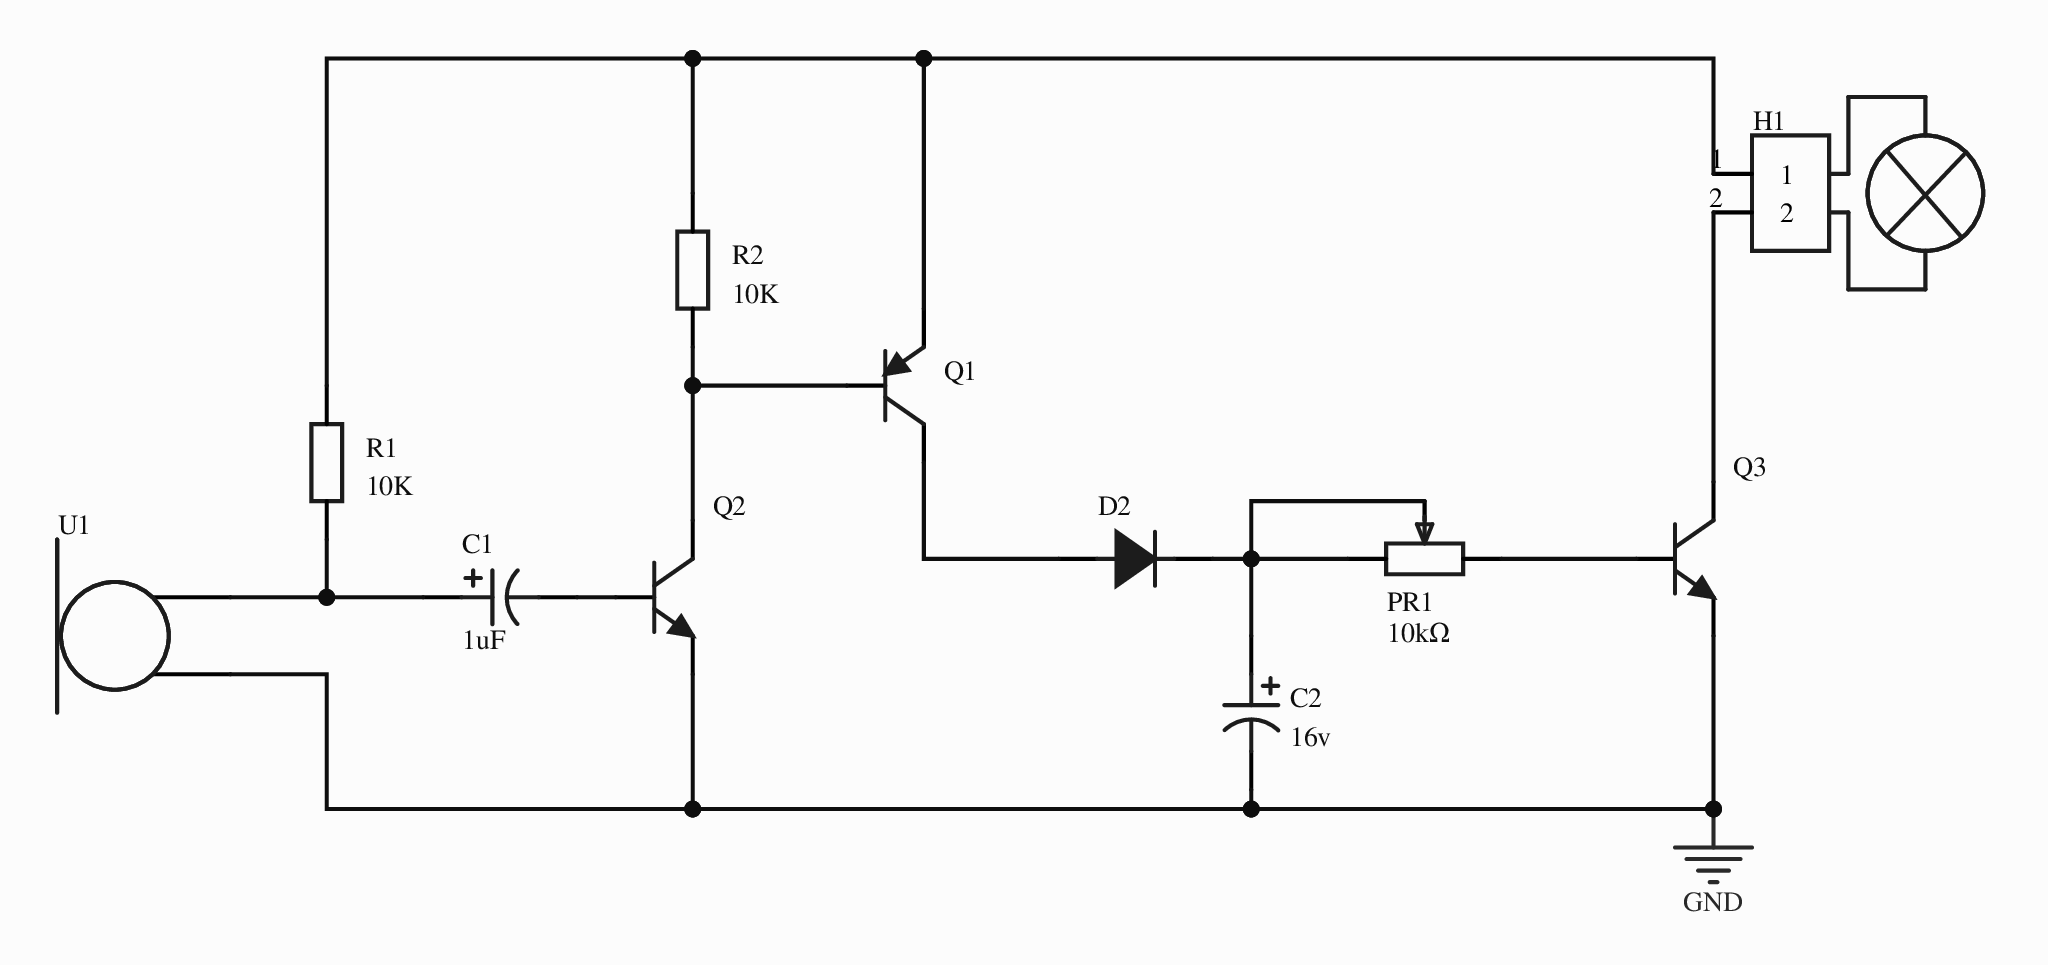
[diagram p0: MISC49923-3.schdoc]
# Altium project MISC49923-2.PrjPcb
1 sheet, 11 parts. Net scope: global (net labels, ports and power ports of the same name join across sheets).
Board file: MISC49923.pcbdoc

## Sheet MISC49923-3.schdoc
size 297 x 209 mm; Version: V1.0; @Project Name: MISC49923; @Update Date: 2026-10-05; @Create Date: 2026-10-05; @Board Name: MISC49923; @Create Time: 20:24:00; @Page Count: 1; @Page No: 1; @Schematic Name: MISC49923; @Update Time: 20:24:00; Size: A4

### Parts
C1  1uF  [CAP-TH_BD5.0-P2.00-D0.8-FD-10UF50VC110GL]
C2  16v  [CAP-TH_BD5.0-P2.00-D0.8-FD-10UF50VC110GL]
D2  (no value)  [SMA_1N4007]
H1  (no value)  [HDR-TH_2P-P2.54-V-M-1]
PR1  10kΩ  [R_3296]
Q1  (no value)  [S8550P_SOT]
Q2  (no value)  [S8050_SOT-23]
Q3  (no value)  [S8050_SOT-23]
R1  10K  [R0603]
R2  10K  [R0603]
U1  Current source  [咪头]  (value not drawn)

### Nets
GND: C2.2 Q2.2 Q3.2 U1.1
NetC1_1: C1.1 R1.1 U1.2
NetC1_2: C1.2 Q2.1
NetC2_1: C2.1 D2.1(K) PR1.2 PR1.3
NetD2_2: D2.2(A) Q1.3(C)
NetH1_1: H1.1 Q1.2(E) R1.2 R2.2
NetH1_2: H1.2 Q3.3
NetPR1_1: PR1.1 Q3.1
NetQ1_1: Q1.1(B) Q2.3 R2.1

### Library data of the parts
C1 C2 = 10UF50VC110GL: Capacitance:10uF;Tolerance:±20%;Rated voltage:50V;Ripple current:120mA@100KHz;Equivalent series resistance(ESR):1.6Ω;; Manufacturer: Econd(米朗电子); AddInBom: yes; ModelId: b35ab6b0460c4c43a629d91cfc2b58780819f05c4eef4c71ace90d822a990e87; ModelTransform: 196.85,196.85,0,0,0,0,0,0,-196.85; Tolerance: ±20%; Voltage Rating: 50V; Equivalent Series Resistance(ESR): 1.6Ω; Pin Spacing: 2mm; Lifetime: 5000hrs@105℃; Symbol: 10UF50VC110GL; Device: 10UF50VC110GL; FootprintName: CAP-TH_BD5.0-P2.00-D0.8-FD-10UF50VC110GL; LCSC Part Name: 10uF ±20% 50V; ManufacturerPart: 10UF50VC110GL; Supplier Footprint: 插件,D5xL11mm; JLCPCB Part Class: Extended Part; Datasheet: https://item.szlcsc.com/datasheet/10UF50VC110GL/49031974.html; Supplier: LCSC; ConvertToPcb: yes; ModelName: CAP-TH_BD5.0-P2.00-D0.8-FD-10UF50VC110GL; Ripple Current: 120mA@100KHz; Diameter: 5mm; Height - Seated (Max): 11mm; Operating Temperature: -40℃~+105℃
  C1: Value: 1uF
  C2: Value: 16v
D2 = D_1N4007: AddInBom: yes; ModelId: 4f1e9ef2303f48b48aa8ce0cacf8d7b10819f05c4eef4c71ace90d822a990e87; ModelName: SMA_L4.4-W2.8-LS5.4-RD; ModelTransform: 204.7,102.4,82.7,0,0,0,0,0,0; Symbol: D_1N4007; Device: D_1N4007; FootprintName: SMA_1N4007; ConvertToPcb: yes; Supplier Footprint: SMA
H1 = HDR-M_2.54_1x2P: Symbol: 210S-1*2P L=11.6MMGold-plated black; ConvertToPcb: yes; ModelId: 79b2e9f2d70a4d68a1b7098f27c6d4c50819f05c4eef4c71ace90d822a990e87; ModelName: HDR-M-2.54_1x2; ModelTransform: 200,100,0,0,0,0,0,0,-118.11; Device: HDR-M_2.54_1x2P; FootprintName: HDR-TH_2P-P2.54-V-M-1; AddInBom: yes; SupplierPart: C124375; Supplier Footprint: 插件
PR1 = R_3296: ConvertToPcb: yes; ModelId: b182808559bb43bda9e7de64b64134cb0819f05c4eef4c71ace90d822a990e87; ModelName: 3296W; ModelTransform: 373.98,188.96,590.49,180,0,0,0,0,-140; Symbol: R_3296; Device: R_3296; FootprintName: R_3296; AddInBom: yes; Supplier Footprint: 直插; Value: 10kΩ
Q1 = S8550_SOT_PNP: Symbol: PNP; 3D Model: 9c0df02d6f3e44e889da37f3e5bf54960819f05c4eef4c71ace90d822a990e87; 3D Model Transform: 98.43,114.17,37.91,0,0,0,0,0,0; ConvertToPcb: yes; ModelName: SOT-23-3_L2.9-W1.4-P1.90-LS2.5-BR; Device: S8550_SOT_PNP; Supplier Footprint: SOT-23; FootprintName: S8550P_SOT; AddInBom: yes
Q2 Q3 = S8050_SOT_NPN: Symbol: NPN; 3D Model: c62791f0466c4ae2a892c056b845b0ca0819f05c4eef4c71ace90d822a990e87; 3D Model Transform: 98.6,114.12,41.29,180,0,0,0,0,-3; ConvertToPcb: yes; ModelName: SOT-23-3P_L2.9-W1.3-H1.0-LS2.4-P0.95; Device: S8050_SOT_NPN; Supplier Footprint: SOT-23; FootprintName: S8050_SOT-23; AddInBom: yes
R1 R2 = Res_0603: Symbol: Resistor; ConvertToPcb: yes; ModelId: fc143cca1e79419f9cd78b61e9279f080819f05c4eef4c71ace90d822a990e87; ModelTransform: 31.8897,63.7794,0,90,0,0,0,0,0; Device: Res_0603; FootprintName: R0603; AddInBom: yes; Supplier Footprint: 0603; ModelName: R0603; Value: 10K
U1 = 咪头: Symbol: Microphone; Add into BOM: yes; Device: Microphone; FootprintName: Microphone; ConvertToPcb: yes